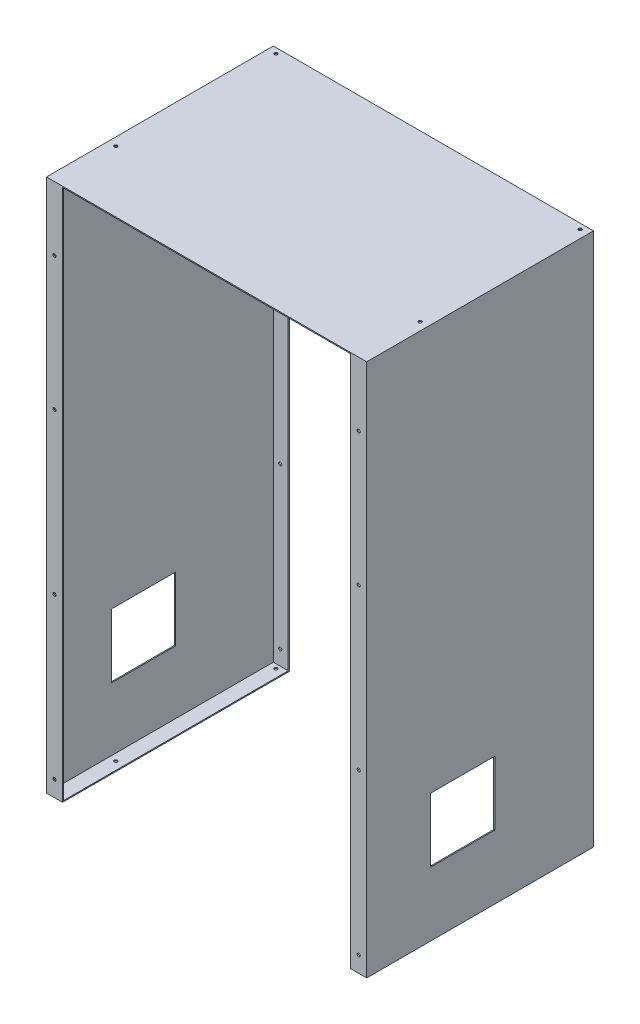
SolidWorks part; units mm, degrees
ref_plane "前视" through (0, 0, 0) normal (0, 0, 1) x (1, 0, 0)
ref_plane "上视" through (0, 0, 0) normal (0, 1, 0) x (1, 0, 0)
ref_plane "右视" through (0, 0, 0) normal (1, 0, 0) x (0, 0, -1)
sketch "草图1" plane through (0, 0, 0) normal (0, 1, 0) x (1, 0, 0)
  line L1 (0, 0) -> (600, 0)
  line L2 (0, 0) -> (0, 425)
  line L3 (0, 425) -> (600, 425)
  line L4 (600, 0) -> (600, 425)
  dimension "D1" = 600
  dimension "D2" = 425
extrude "凸台-拉伸1" add sketch "草图1" along normal blind 1000
shell "抽壳2" thickness 2
sketch "草图2" plane through (0, 0, 0) normal (0, 0, 1) x (1, 0, 0)
  line L0 (0, 0) -> (600, 0) construction
  line L1 (30, 0) -> (570, 0)
  line L2 (30, 0) -> (30, 998)
  line L3 (30, 998) -> (570, 998)
  line L4 (570, 0) -> (570, 998)
  line L5 (0, 1000) -> (0, 0) construction
  line L6 (0, 1000) -> (600, 1000) construction
  line L7 (600, 1000) -> (600, 0) construction
  dimension "D1" = 30
  dimension "D2" = 2
  dimension "D3" = 30
extrude "切除-拉伸1" cut sketch "草图2" against normal blind 900
sketch "草图5" plane through (0, 0, 0) normal (0, -1, 0) x (1, 0, 0)
  line L1 (2, -2) -> (30, -2)
  line L2 (2, -2) -> (2, -423)
  line L3 (2, -423) -> (30, -423)
  line L4 (30, -2) -> (30, -423)
  line L5 (598, -2) -> (570, -2)
  line L6 (598, -2) -> (598, -423)
  line L7 (598, -423) -> (570, -423)
  line L8 (570, -2) -> (570, -423)
extrude "凸台-拉伸2" add sketch "草图5" against normal blind 2
sketch "草图6" plane through (600, 0, 0) normal (1, 0, 0) x (0, 0, -1)
  line L0 (0, 0) -> (425, 0) construction
  line L1 (120, 240) -> (240, 240)
  line L2 (120, 240) -> (120, 120)
  line L3 (120, 120) -> (240, 120)
  line L4 (240, 240) -> (240, 120)
  line L5 (0, 1000) -> (0, 0) construction
  dimension "D1" = 120
  dimension "D2" = 120
  dimension "D3" = 120
  dimension "D4" = 120
extrude "切除-拉伸3" cut sketch "草图6" against normal blind 812
sketch "草图7" plane through (0, 0, 0) normal (0, -1, 0) x (1, 0, 0)
  line L0 (15, -507.93) -> (15, -115) construction
  line L1 (0, 0) -> (30, 0) construction
  line L2 (0, -425) -> (0, 0) construction
  line L3 (300, 0) -> (300, -476.0843) construction
  line L4 (570, 0) -> (30, 0) construction
  circle A0 centre (15, -115) radius 3
  circle A1 centre (585, -415) radius 3
  circle A3 centre (15, -415) radius 3
  circle A5 centre (585, -115) radius 3
  dimension "D1" = 6
  dimension "D2" = 115
  dimension "D3" = 300
  dimension "D4" = 6
  dimension "D6" = 15
extrude "切除-拉伸4" cut sketch "草图7" against normal blind 1118
sketch "草图8" plane through (0, 0, -425) normal (0, 0, -1) x (-1, 0, 0)
  line L0 (-15, 30) -> (-15, 1025.106) construction
  line L1 (-30, 0) -> (0, 0) construction
  line L2 (0, 1000) -> (0, 0) construction
  line L3 (-300, 998) -> (-300, -80.7181) construction
  line L4 (-570, 998) -> (-30, 998) construction
  circle A0 centre (-15, 30) radius 3
  circle A1 centre (-15, 330) radius 3
  circle A2 centre (-15, 630) radius 3
  circle A3 centre (-585, 30) radius 3
  circle A4 centre (-585, 330) radius 3
  circle A5 centre (-15, 880) radius 3
  circle A6 centre (-585, 630) radius 3
  circle A7 centre (-585, 880) radius 3
  dimension "D1" = 30
  dimension "D3" = 6
  dimension "D4" = 6
  dimension "D5" = 300
  dimension "D6" = 6
  dimension "D7" = 300
  dimension "D8" = 6
  dimension "D9" = 250
  dimension "D2" = 15
extrude "切除-拉伸5" cut sketch "草图8" against normal blind 671
